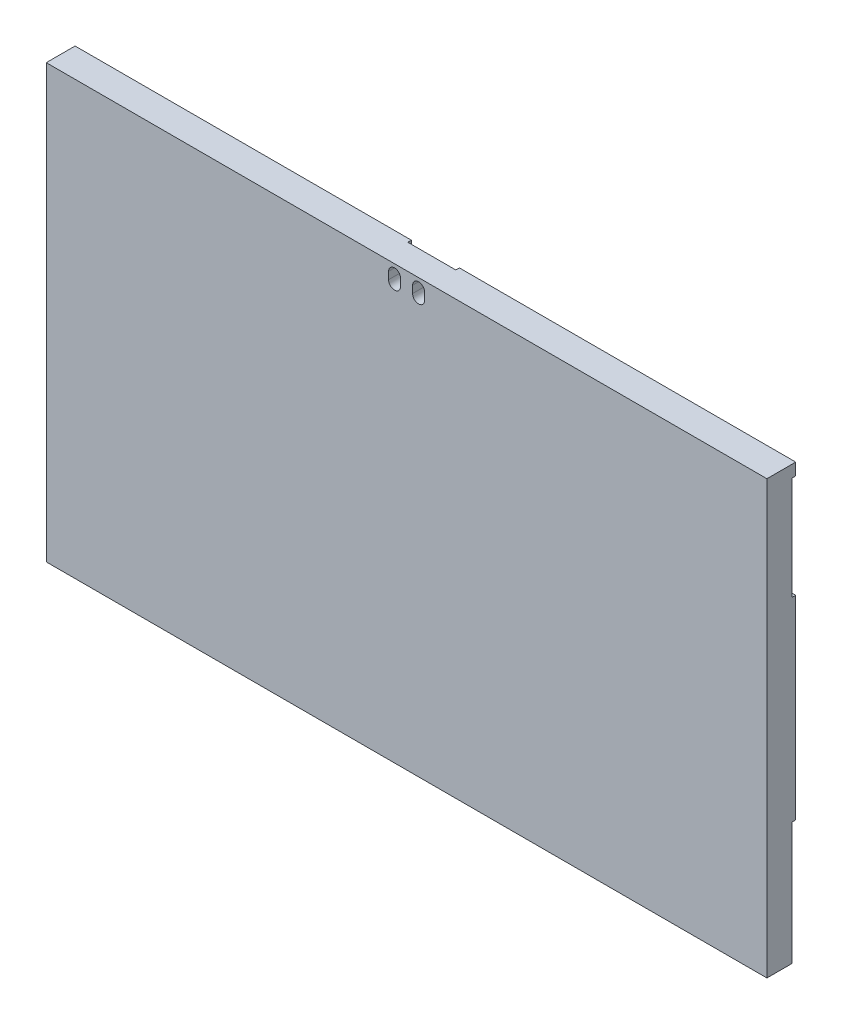
from build123d import *

# Parameters (mm, degrees)
SKETCH_1_W          = 300
SKETCH_1_H          = 180
EXTRUDE_1_DEPTH     = 12
SKETCH_2_W          = 300
SKETCH_2_H          = 43
SKETCH_2_H_2        = 51
CUT_EXTRUDE_1_DEPTH = 1.5
SKETCH_3_W          = 20
SKETCH_3_H          = 5
CUT_EXTRUDE_2_DEPTH = 1.5
CUT_EXTRUDE_3_REACH = 177.243


with BuildPart() as part:
    # 草图1 → 凸台-拉伸1 (new body)
    with BuildSketch(Plane.XY):
        Rectangle(SKETCH_1_W, SKETCH_1_H)
    extrude(amount=EXTRUDE_1_DEPTH)

    # 草图2 → 切除-拉伸1 (cut)
    with BuildSketch(Plane(origin=(0, 0, 0), x_dir=(-1, 0, 0), z_dir=(0, 0, -1))):
        with Locations((0, 63.5)):
            Rectangle(SKETCH_2_W, SKETCH_2_H)
        with Locations((0, -64.5)):
            Rectangle(SKETCH_2_W, SKETCH_2_H_2)
    extrude(amount=-CUT_EXTRUDE_1_DEPTH, mode=Mode.SUBTRACT)

    # 草图3 → 切除-拉伸2 (cut)
    with BuildSketch(Plane(origin=(0, 0, 0), x_dir=(-1, 0, 0), z_dir=(0, 0, -1))):
        with Locations((0, 87.5)):
            Rectangle(SKETCH_3_W, SKETCH_3_H)
    extrude(amount=-CUT_EXTRUDE_2_DEPTH, mode=Mode.SUBTRACT)

    # 草图4 → 切除-拉伸3 (cut, up to next)
    with BuildSketch(Plane(origin=(0, 0, 1.5), x_dir=(-1, 0, 0), z_dir=(0, 0, -1)), mode=Mode.PRIVATE) as cut_extrude_3_sk1:
        with BuildLine():
            Line((-7.5, 83), (-7.5, 86))
            ThreePointArc((-7.5, 86), (-5, 88.5), (-2.5, 86))
            Line((-2.5, 86), (-2.5, 83))
            ThreePointArc((-2.5, 83), (-5, 80.5), (-7.5, 83))
        make_face()
    cut_extrude_3_tool1 = extrude(cut_extrude_3_sk1.sketch, amount=-CUT_EXTRUDE_3_REACH, mode=Mode.PRIVATE) & part.part
    cut_extrude_3 = cut_extrude_3_tool1.solids().sort_by_distance((5, 84.5, 1.5))[0]
    add(cut_extrude_3, mode=Mode.SUBTRACT)

    # 镜向1: 切除-拉伸3 across plane
    add(cut_extrude_3.mirror(Plane(origin=(0, 0, 0), x_dir=(0, 0, 1), z_dir=(1, 0, 0))), mode=Mode.SUBTRACT)


solid = part.part
